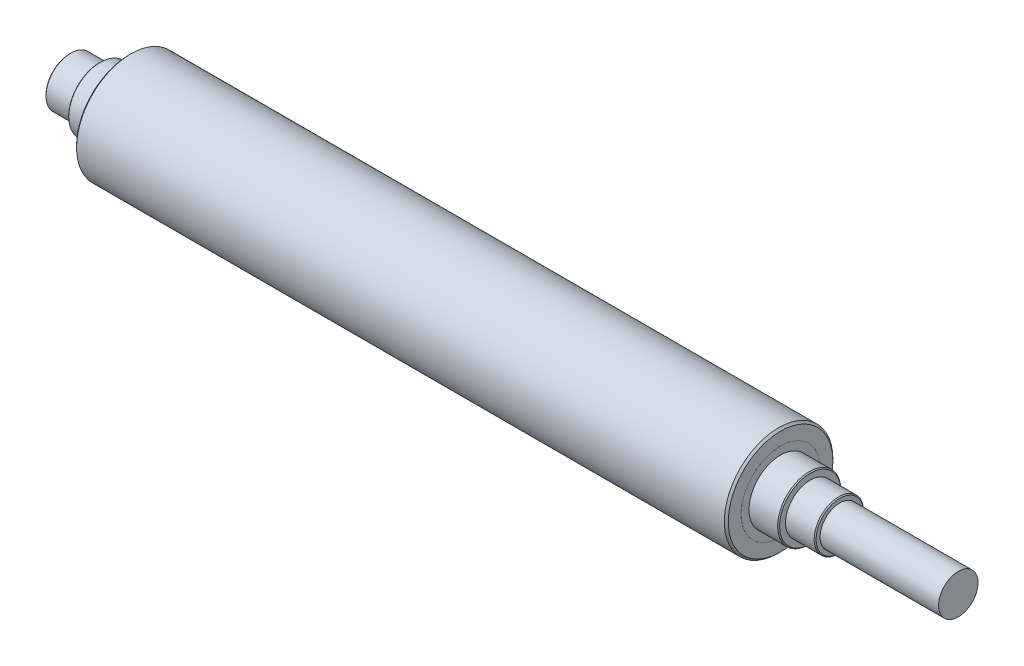
SolidWorks part; units mm, degrees
ref_plane "Front Plane" through (0, 0, 0) normal (0, 0, 1) x (1, 0, 0)
ref_plane "Top Plane" through (0, 0, 0) normal (0, 1, 0) x (1, 0, 0)
ref_plane "Right Plane" through (0, 0, 0) normal (1, 0, 0) x (0, 0, -1)
sketch "Sketch1" plane through (0, 0, 0) normal (0, 0, 1) x (1, 0, 0)
  line L0 (0, 0) -> (388.5641, 0) construction
  line L2 (450, 10) -> (390, 10)
  line L3 (0, 0) -> (0, 12.5)
  line L4 (0, 12.5) -> (15, 12.5)
  line L7 (15, 12.5) -> (15, 16)
  line L8 (15, 16) -> (30, 16)
  line L9 (390, 10) -> (390, 12.5)
  line L11 (30, 16) -> (30, 20)
  line L12 (30, 20) -> (360, 20)
  line L13 (360, 16) -> (360, 20)
  line L16 (360, 16) -> (375, 16)
  line L17 (375, 12.5) -> (375, 16)
  line L18 (0, 0) -> (450, 0)
  line L20 (375, 12.5) -> (390, 12.5)
  line L21 (450, 0) -> (450, 10)
  dimension "D1" = 25
  dimension "D2" = 40
  dimension "D3" = 32
  dimension "D4" = 15
  dimension "D5" = 15
  dimension "D6" = 330
  dimension "D7" = 15
  dimension "D8" = 15
  dimension "D9" = 60
  dimension "D10" = 20
revolve "Revolve1" add sketch "Sketch1" angle 360 about L0
sketch "Sketch2" plane through (360, 0, 0) normal (1, 0, 0) x (0, 0, -1)
  circle A0 centre (0, 0) radius 20
  circle A1 centre (0, 0) radius 27.5
  dimension "D1" = 55
extrude "Boss-Extrude1" add sketch "Sketch2" against normal up to surface (330 mm away) separate body up to face at (30, 0, 16)
chamfer "Chamfer1" distance 0.5 angle 45 4 edges at (0, 0, 12.5) (15, 0, 16) (375, 0, 16) (390, 0, 12.5)
chamfer "Chamfer2" distance 1 angle 45 2 edges at (360, 0, -27.5) (30, 0, -27.5)
